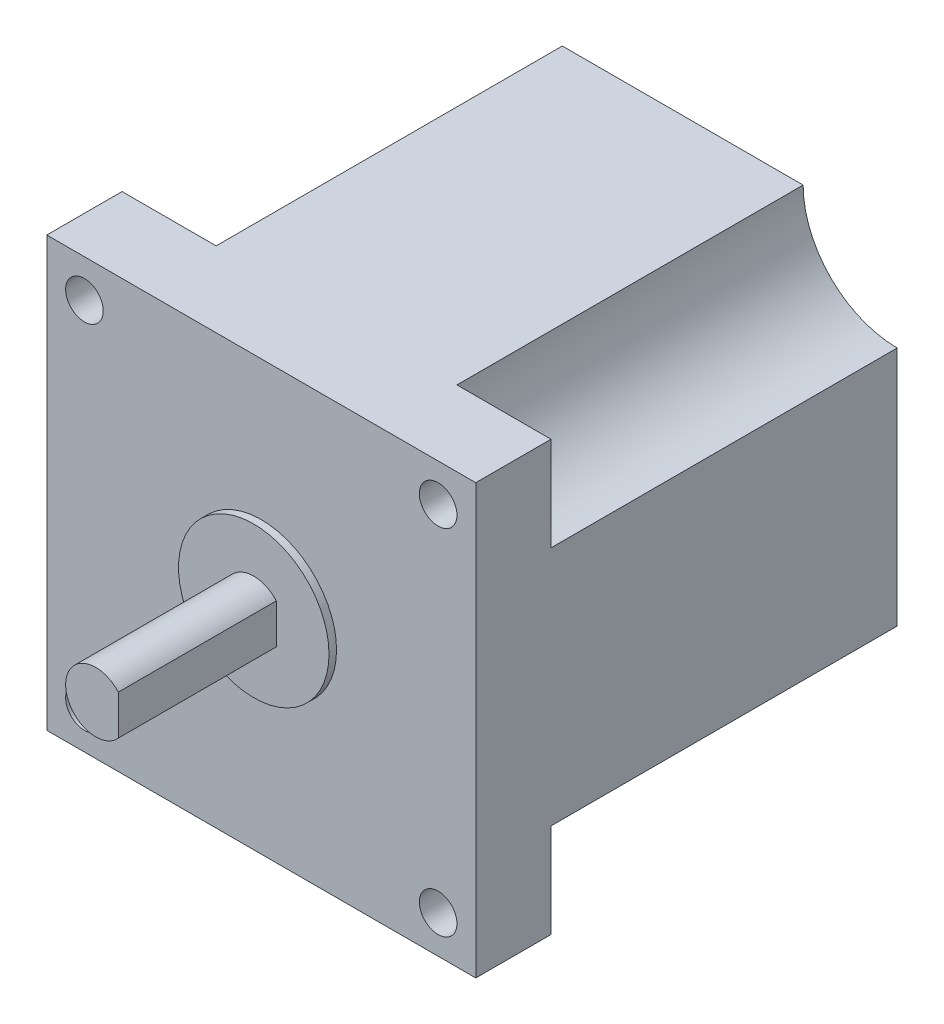
from build123d import *

# Parameters (mm, degrees)
SKETCH1_W           = 57
SKETCH1_H           = 57
BOSS_EXTRUDE1_DEPTH = 56
SKETCH2_R           = 2.5
CUT_EXTRUDE1_DEPTH  = 98
SKETCH4_R           = 10
BOSS_EXTRUDE2_DEPTH = 1
SKETCH5_R           = 4
BOSS_EXTRUDE3_DEPTH = 21
CUT_EXTRUDE2_DEPTH  = 21
SKETCH7_R           = 12.5
CUT_EXTRUDE3_DEPTH  = 46


with BuildPart() as part:
    # Sketch1 → Boss-Extrude1 (new body)
    with BuildSketch(Plane.XY):
        Rectangle(SKETCH1_W, SKETCH1_H)
    extrude(amount=BOSS_EXTRUDE1_DEPTH)

    # Sketch2 → Cut-Extrude1 (cut)
    with BuildSketch(Plane.XY.offset(56)):
        with Locations((-23.5, 23.5)):
            Circle(SKETCH2_R)
        with Locations((23.5, 23.5)):
            Circle(SKETCH2_R)
        with Locations((23.5, -23.5)):
            Circle(SKETCH2_R)
        with Locations((-23.5, -23.5)):
            Circle(SKETCH2_R)
    extrude(amount=-CUT_EXTRUDE1_DEPTH, mode=Mode.SUBTRACT)

    # Sketch4 → Boss-Extrude2 (add)
    with BuildSketch(Plane.XY.offset(56)):
        Circle(SKETCH4_R)
    extrude(amount=BOSS_EXTRUDE2_DEPTH)

    # Sketch5 → Boss-Extrude3 (add)
    with BuildSketch(Plane.XY.offset(57)):
        with Locations(Location((0, 0, 0), (0, 0, 180))):
            Circle(SKETCH5_R)
    extrude(amount=BOSS_EXTRUDE3_DEPTH)

    # Sketch6 → Cut-Extrude2 (cut)
    with BuildSketch(Plane.XY.offset(78)):
        Polygon((3, 101.241638907), (3, 2.645751311), (3, -2.645751311), (3, -101.241638907), (200.191775192, -101.241638907), (200.191775192, 101.241638907), align=None)
    extrude(amount=-CUT_EXTRUDE2_DEPTH, mode=Mode.SUBTRACT)

    # Sketch7 → Cut-Extrude3 (cut)
    with BuildSketch(Plane(origin=(0, 0, 0), x_dir=(-1, 0, 0), z_dir=(0, 0, -1))):
        with Locations((-28.5, 28.5)):
            Circle(SKETCH7_R)
        with Locations((28.5, 28.5)):
            Circle(SKETCH7_R)
        with Locations((28.5, -28.5)):
            Circle(SKETCH7_R)
        with Locations((-28.5, -28.5)):
            Circle(SKETCH7_R)
    extrude(amount=-CUT_EXTRUDE3_DEPTH, mode=Mode.SUBTRACT)


solid = part.part
